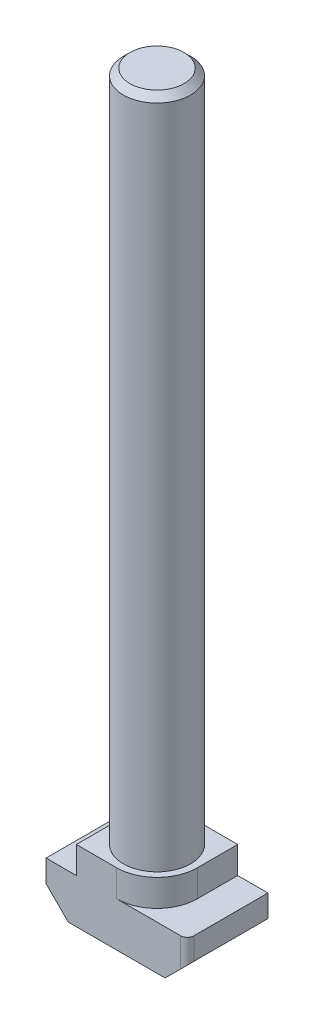
SolidWorks part; units mm, degrees
ref_plane "Front Plane" through (0, 0, 0) normal (0, 0, 1) x (1, 0, 0)
ref_plane "Top Plane" through (0, 0, 0) normal (0, 1, 0) x (1, 0, 0)
ref_plane "Right Plane" through (0, 0, 0) normal (1, 0, 0) x (0, 0, -1)
ref_plane "Plane1" through (0, 0, -3) normal (0, 0, -1) x (-1, 0, 0)
sketch "Sketch1" plane through (0, 0, -3) normal (0, 0, -1) x (-1, 0, 0)
  line L0 (5.25, 2) -> (-5.25, 2)
  line L1 (-5.25, 2) -> (-5.25, -1.65)
  line L2 (-5.25, -1.65) -> (-3.6, -3.3)
  line L3 (-3.6, -3.3) -> (3.6, -3.3)
  line L4 (3.6, -3.3) -> (5.25, -1.65)
  line L5 (5.25, -1.65) -> (5.25, 2)
extrude "Boss-Extrude1" add sketch "Sketch1" against normal blind 6
sketch "Sketch2" plane through (0, 0, 3) normal (0, 0, 1) x (1, 0, 0)
  line L0 (-5.25, 0) -> (-3, 0)
  line L1 (-3, 0) -> (-3, 2)
  line L2 (-3, 2) -> (-5.25, 2)
  line L3 (-5.25, 2) -> (-5.25, 0)
extrude "Cut-Extrude1" cut sketch "Sketch2" against normal through all
sketch "Sketch3" plane through (0, 0, 3) normal (0, 0, 1) x (1, 0, 0)
  line L0 (3, 0) -> (5.25, 0)
  line L1 (5.25, 0) -> (5.25, 2)
  line L2 (5.25, 2) -> (3, 2)
  line L3 (3, 2) -> (3, 0)
extrude "Cut-Extrude2" cut sketch "Sketch3" against normal through all
ref_plane "Plane2" through (0, 0, 0) normal (0, 0, -1) x (-1, 0, 0)
sketch "Sketch4" plane through (0, 0, 0) normal (0, 0, -1) x (-1, 0, 0)
  line L0 (-2.5, 2) -> (0, 2)
  line L1 (0, 2) -> (0, 52)
  line L2 (0, 52) -> (-2.5, 52)
  line L3 (-2.5, 52) -> (-2.5, 2)
  line L4 (0, 2) -> (0, 52) construction
  dimension "D1" = 50
revolve "Revolve1" add sketch "Sketch4" angle 360 about L4
chamfer "Chamfer1" distance 0.4905 angle 45 1 edges at (-2.5, 52, 0)
fillet "Fillet1" radius 0.5 2 edges at (-5.25, -0.825, -3) (5.25, -0.825, 3)
fillet "Fillet2" radius 3 2 edges at (3, 1, 3) (-3, 1, -3)
